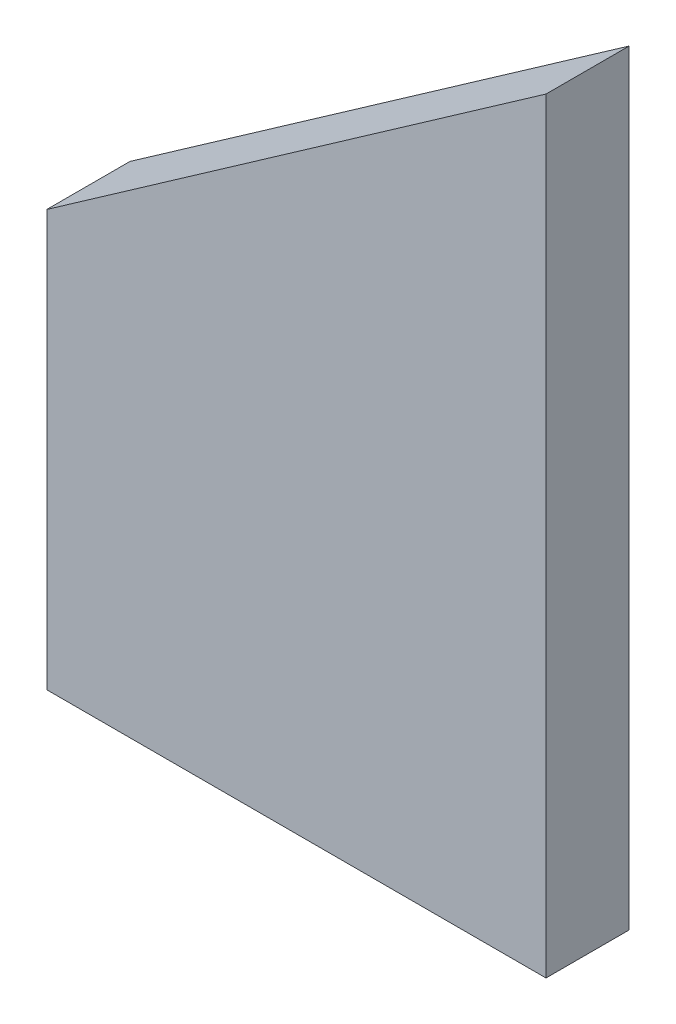
from build123d import *

# Parameters (mm, degrees)
EXTRUDE_START   = -260
EXTRUDE_1_DEPTH = 12


with BuildPart() as part:
    # 草图1 → 凸台-拉伸1 (new body)
    with BuildSketch(Plane.XY.offset(EXTRUDE_START)):
        Polygon((-102, 125.580906485), (-102, 185.580906485), (-30, 235.995849236), (-30, 125.580906485), align=None)
    extrude(amount=EXTRUDE_1_DEPTH)


solid = part.part
